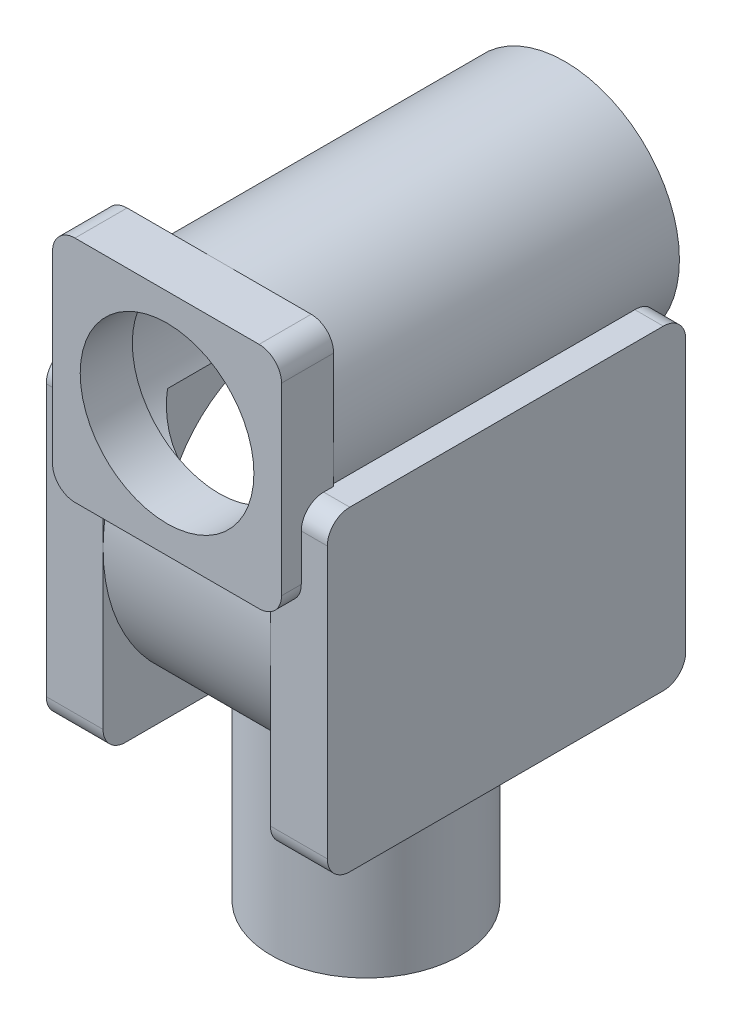
from build123d import *
from build123d.topology import SkipClean

# Parameters (mm, degrees)
SKETCH1_R                       = 72.5
BOSS_EXTRUDE1_DEPTH             = 252
SKETCH2_W                       = 145
SKETCH2_H                       = 145
BOSS_EXTRUDE2_DEPTH             = 33
BOSS_EXTRUDE3_DEPTH             = 53
BOSS_EXTRUDE3_DEPTH_BACK        = 53
SKETCH7_R                       = 113.5
SKETCH7_R_2                     = 99
SKETCH8_W                       = 227
SKETCH8_H                       = 200
BOSS_EXTRUDE4_DEPTH             = 36
SKETCH10_W                      = 227
SKETCH10_H                      = 200
BOSS_EXTRUDE5_DEPTH             = 36
SKETCH12_R                      = 75
CUT_EXTRUDE4_DEPTH              = 36
CUT_EXTRUDE1_DEPTH              = 93
CUT_EXTRUDE1_DEPTH_BACK         = 93
SKETCH3_R                       = 63
SKETCH5_R                       = 55
CUT_EXTRUDE3_DEPTH              = 33
SKETCH13_R                      = 75
CUT_EXTRUDE5_DEPTH              = 28
SKETCH15_R                      = 99
CUT_EXTRUDE6_DEPTH              = 106
CUT_EXTRUDE2_START              = -33
SKETCH4_R                       = 55
CUT_EXTRUDE2_DEPTH              = 33
BOSS_EXTRUDE6_REACH             = 394.391
BOSS_EXTRUDE6_END_RADIUS        = 113.5
SKETCH18_R                      = 60
SKETCH18_R_2                    = 40
BOSS_EXTRUDE6_DIRECTION_2_DEPTH = 110
BOSS_EXTRUDE7_START             = -7.282064
SKETCH19_R                      = 40
BOSS_EXTRUDE7_DEPTH             = 42.782064
FILLET1_R                       = 14.2


with BuildPart() as part:
    # Sketch1 → Boss-Extrude1 (new body)
    with BuildSketch(Plane.XY):
        Circle(SKETCH1_R)
    extrude(amount=BOSS_EXTRUDE1_DEPTH)

    # Sketch2 → Boss-Extrude2 (add)
    with BuildSketch(Plane.XY.offset(252)):
        Rectangle(SKETCH2_W, SKETCH2_H)
    extrude(amount=-BOSS_EXTRUDE2_DEPTH)

    # Sketch7 → Boss-Extrude3 (add, two sides: drawn at the far end of the back side and taken through both)
    with BuildSketch(Plane(origin=(0, 0, 0), x_dir=(0, 0, -1), z_dir=(1, 0, 0)).offset(-BOSS_EXTRUDE3_DEPTH_BACK)):
        with Locations((-126, -101.308)):
            Circle(SKETCH7_R)
        with Locations((-126, -101.308)):
            Circle(SKETCH7_R_2, mode=Mode.SUBTRACT)
    extrude(amount=BOSS_EXTRUDE3_DEPTH + BOSS_EXTRUDE3_DEPTH_BACK)

    # Sketch8 → Boss-Extrude4 (add)
    with BuildSketch(Plane(origin=(53, 0, 0), x_dir=(0, 0, -1), z_dir=(1, 0, 0))):
        with Locations((-126, -114.808)):
            Rectangle(SKETCH8_W, SKETCH8_H)
    extrude(amount=BOSS_EXTRUDE4_DEPTH)

    # Sketch10 → Boss-Extrude5 (add)
    with BuildSketch(Plane.ZY.offset(53)):
        with Locations((126, -114.808)):
            Rectangle(SKETCH10_W, SKETCH10_H)
    extrude(amount=BOSS_EXTRUDE5_DEPTH)

    # Sketch12 → Cut-Extrude4 (cut)
    with BuildSketch(Plane.ZY.offset(89)):
        with Locations((126, -114.808)):
            Circle(SKETCH12_R)
    extrude(amount=-CUT_EXTRUDE4_DEPTH, mode=Mode.SUBTRACT)

    # Sketch3 → Cut-Extrude1 (cut, two sides: drawn at the far end of the back side and taken through both)
    with BuildSketch(Plane.XY.offset(126).offset(-CUT_EXTRUDE1_DEPTH_BACK)):
        with Locations(Location((0, 0, 0), (0, 0, 180))):
            Circle(SKETCH3_R)
    extrude(amount=CUT_EXTRUDE1_DEPTH + CUT_EXTRUDE1_DEPTH_BACK, mode=Mode.SUBTRACT)

    # Sketch5 → Cut-Extrude3 (cut)
    with BuildSketch(Plane(origin=(0, 0, 0), x_dir=(-1, 0, 0), z_dir=(0, 0, -1))):
        Circle(SKETCH5_R)
    extrude(amount=-CUT_EXTRUDE3_DEPTH, mode=Mode.SUBTRACT)

    # Sketch13 → Cut-Extrude5 (cut)
    with BuildSketch(Plane.ZY.offset(-53)):
        with Locations((126, -114.808)):
            Circle(SKETCH13_R)
    extrude(amount=-CUT_EXTRUDE5_DEPTH, mode=Mode.SUBTRACT)

    # Sketch15 → Cut-Extrude6 (cut)
    with SkipClean():  # the faces are left unmerged after this step: merging them gives an invalid solid
        with BuildSketch(Plane.ZY.offset(-53)):
            with Locations((126, -101.308)):
                Circle(SKETCH15_R)
        extrude(amount=CUT_EXTRUDE6_DEPTH, mode=Mode.SUBTRACT)

    # Sketch4 → Cut-Extrude2 (cut)
    with SkipClean():  # the faces are left unmerged after this step: merging them gives an invalid solid
        with BuildSketch(Plane.XY.offset(252).offset(CUT_EXTRUDE2_START)):
            with Locations(Location((0, 0, 0), (0, 0, 180))):
                Circle(SKETCH4_R)
        extrude(amount=CUT_EXTRUDE2_DEPTH, mode=Mode.SUBTRACT)

    # Boss-Extrude6: up to this cylinder (the profile starts outside it)
    with SkipClean():  # the faces are left unmerged after this step: merging them gives an invalid solid
        boss_extrude6_end = Plane(origin=(-51.500934, -101.308, 126), z_dir=(1, 0, 0)) * Cylinder(BOSS_EXTRUDE6_END_RADIUS, 1016.782, mode=Mode.PRIVATE)
        # Sketch18 → Boss-Extrude6 (add, up to the surface)
        with BuildSketch(Plane.XZ.offset(214.808), mode=Mode.PRIVATE) as boss_extrude6_sk1:
            with Locations(Location((0, 126, 0), (0, 0, 27.952886589))):
                Circle(SKETCH18_R)
            with Locations(Location((0, 126, 0), (0, 0, 90))):
                Circle(SKETCH18_R_2, mode=Mode.SUBTRACT)
        boss_extrude6_tool1 = extrude(boss_extrude6_sk1.sketch, amount=-BOSS_EXTRUDE6_REACH, mode=Mode.PRIVATE) - boss_extrude6_end
        add(boss_extrude6_tool1.solids().sort_by_distance((-51.500934, -214.808, 98.670765))[0])
        add(boss_extrude6_tool1.solids().sort_by_distance((-51.500934, -214.808, 98.670765))[1])

    # Sketch18 → Boss-Extrude6 direction 2 (add)
    with BuildSketch(Plane.XZ.offset(214.808)):
        with Locations(Location((0, 126, 0), (0, 0, 27.952886589))):
            Circle(SKETCH18_R)
        with Locations(Location((0, 126, 0), (0, 0, 90))):
            Circle(SKETCH18_R_2, mode=Mode.SUBTRACT)
    extrude(amount=BOSS_EXTRUDE6_DIRECTION_2_DEPTH)

    # Sketch19 → Boss-Extrude7 (add)
    with SkipClean():  # the faces are left unmerged after this step: merging them gives an invalid solid
        with BuildSketch(Plane.XZ.offset(214.808).offset(BOSS_EXTRUDE7_START)):
            with Locations(Location((0, 126, 0), (0, 0, 270))):
                Circle(SKETCH19_R)
        extrude(amount=BOSS_EXTRUDE7_DEPTH)

    # Fillet1
    fillet1_edges = [part.edges().sort_by_distance(p)[0] for p in [
        (-72.5, 72.5, 235.5),
        (72.5, 72.5, 235.5),
        (72.5, -72.5, 245.75),
        (79.985818069, -14.808, 12.5),
        (71, -214.808, 12.5),
        (80.75, -14.808, 239.5),
        (71, -214.808, 239.5),
        (-72.5, -72.5, 245.75),
        (-80.75, -14.808, 239.5),
        (-79.985818069, -14.808, 12.5),
        (-71, -214.808, 239.5),
        (-71, -214.808, 12.5),
    ]]
    fillet(fillet1_edges, radius=FILLET1_R)


solid = part.part
